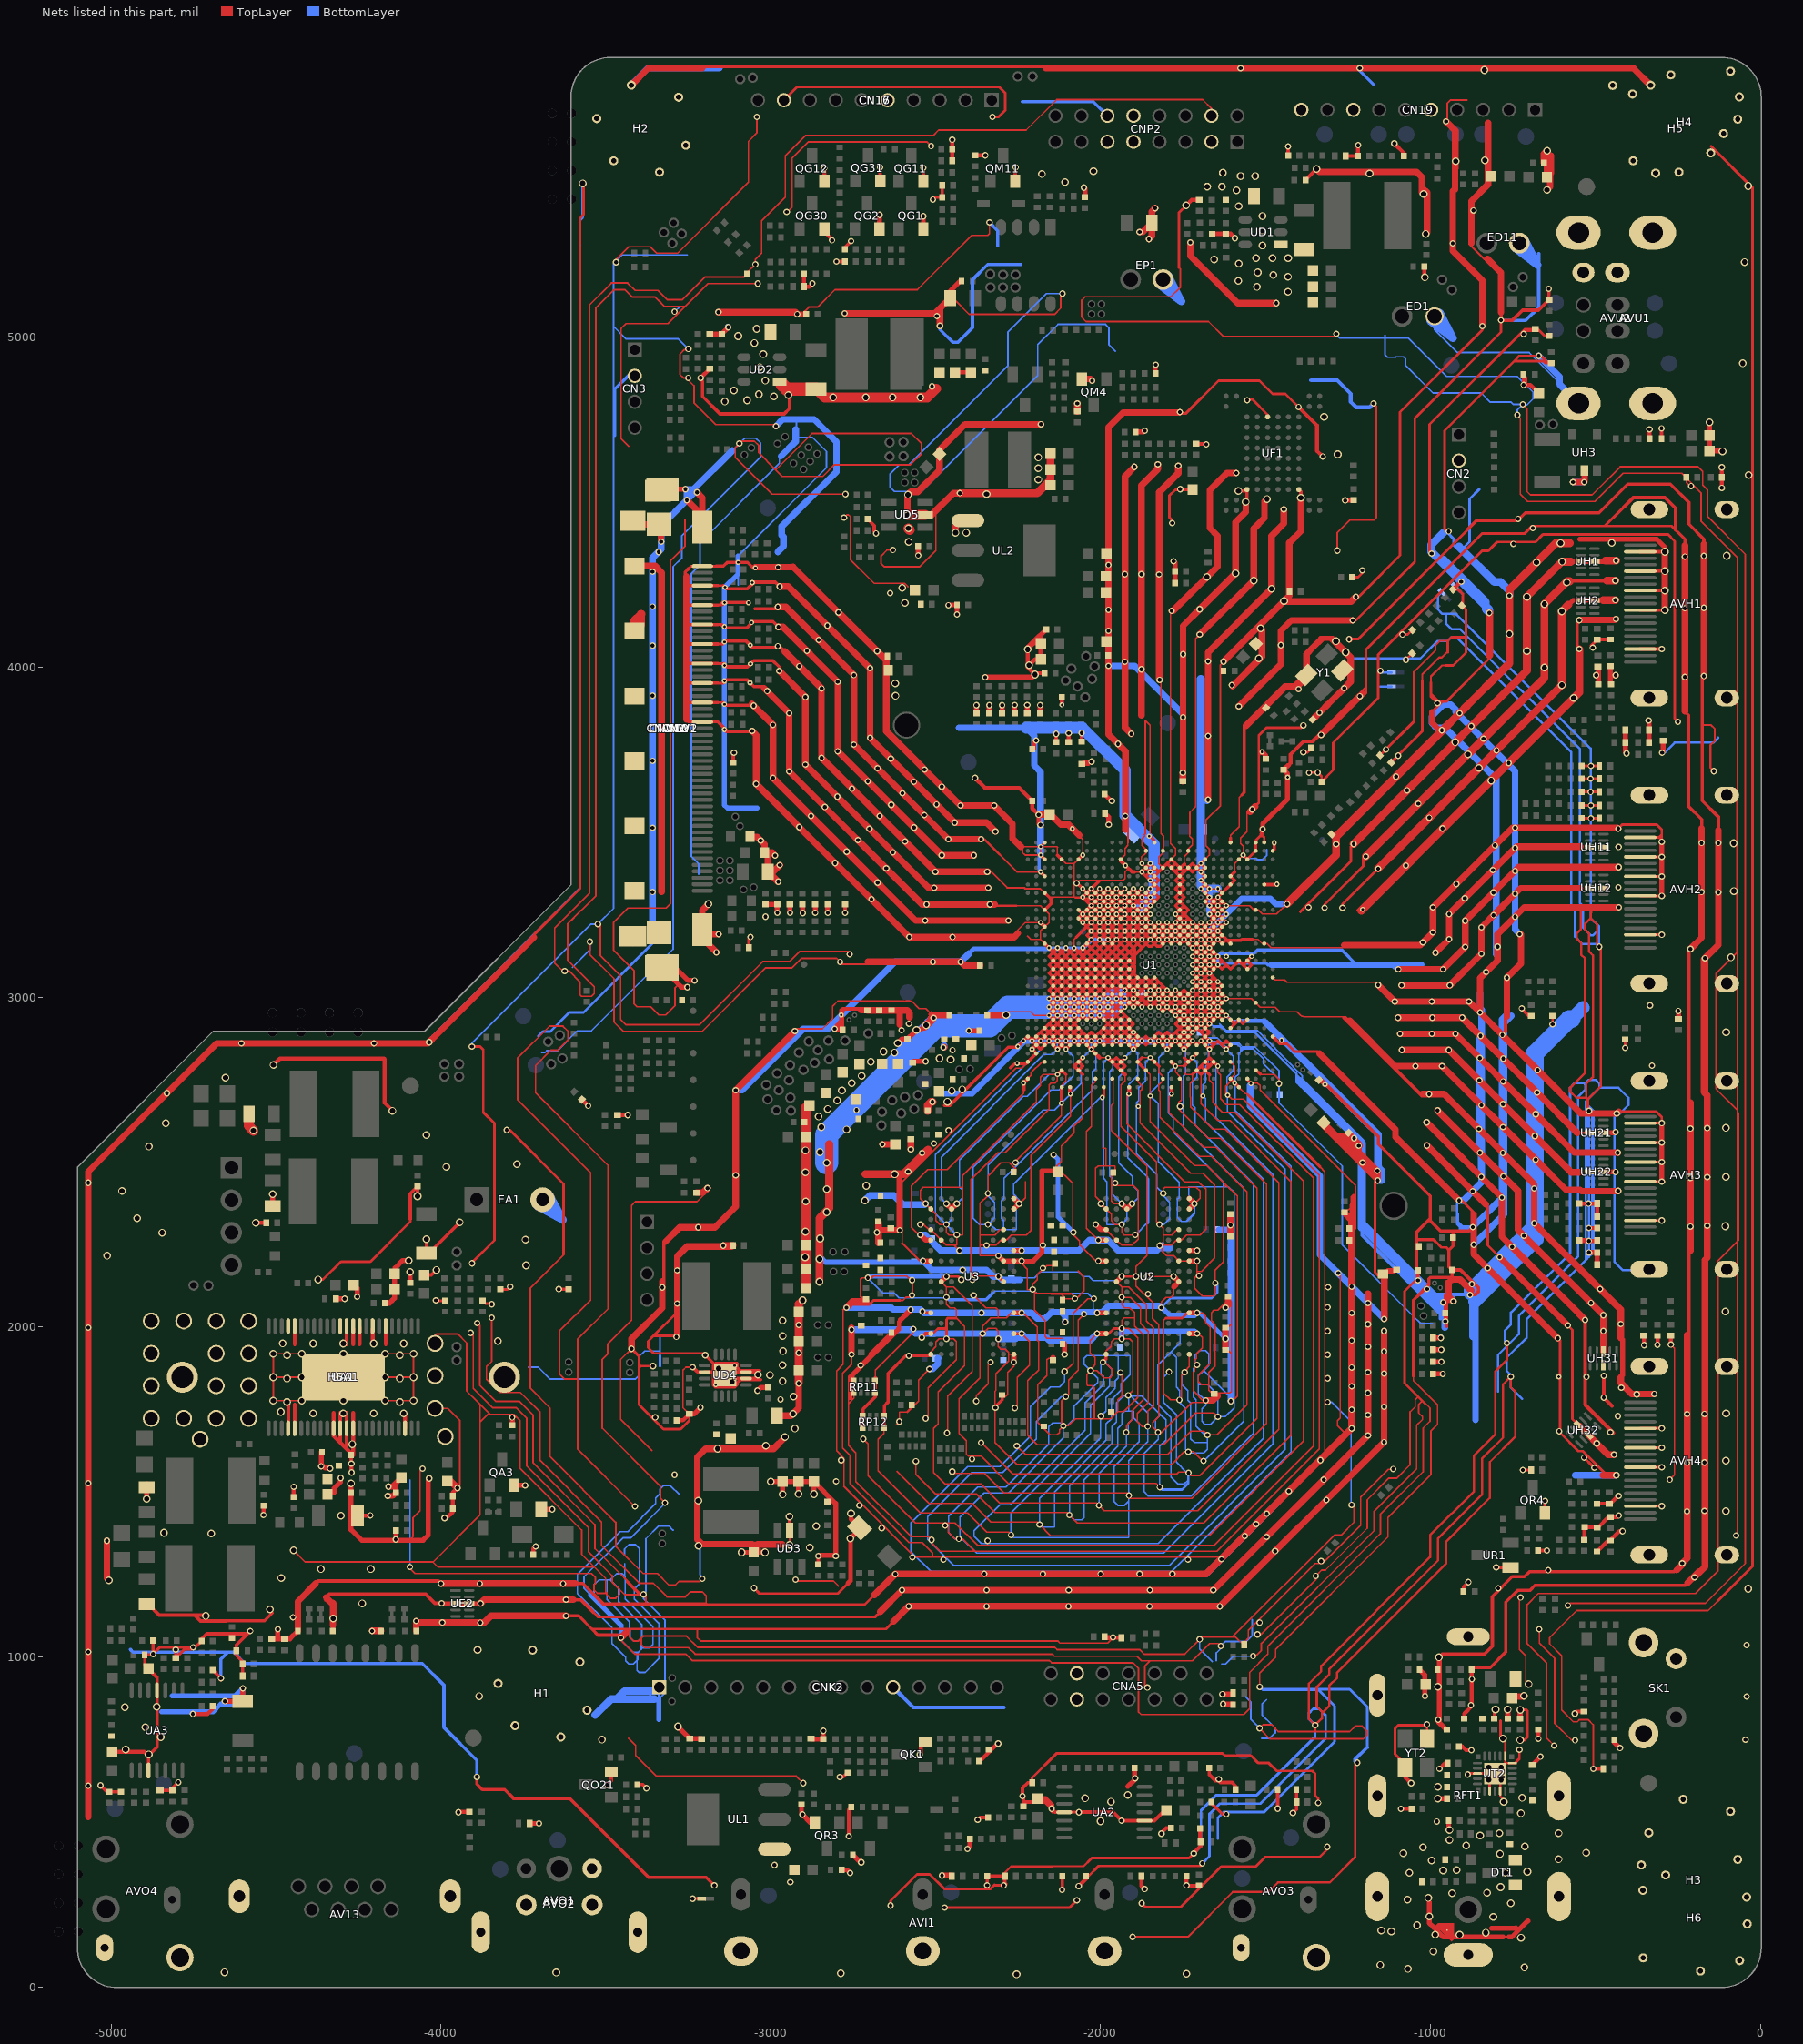
[diagram p0: the nets of this part, all layers, seen from the top]
# Altium PCB MISC86290.PcbDoc (part 19 of 31)
Units mil, origin at the board's own origin, x right, y up, seen from the top; angles counter-clockwise.
Board outline 5104.71 x 5851.49 mil, 2 copper layers (TopLayer, BottomLayer), stack 61.855 mil thick; 1026 components, 667 nets, 4280 pads, 2294 vias.

## Via types
v1: diameter 19.68, hole 11.81, TopLayer to BottomLayer, tented both sides, 1189 vias
v2: diameter 19.68/19.68 (per signal layer), hole 11.81, TopLayer to BottomLayer, tented both sides, 366 vias
v3: diameter 15.75, hole 7.87, TopLayer to BottomLayer, tented both sides, 348 vias
v4: diameter 23.62, hole 15.75, TopLayer to BottomLayer, tented both sides, 309 vias
v5: diameter 15.75/15.75 (per signal layer), hole 7.87, TopLayer to BottomLayer, tented both sides, 59 vias
v6: diameter 24/24 (per signal layer), hole 16, TopLayer to BottomLayer, tented both sides, 23 vias

## Nets (pads, with @x,y where several pads share a name; then routed paths per layer and width w, separated by ;. In a path a pad name is that pad's centre, name@x,y a point inside that pad or via, vN(x,y) a via of type N, cw(c..) or ccw(c..) an arc to the next point about the centre after c; other vN are vias at no path point) (continued)
GND: (continued)
  TopLayer w20: -5069.17,514.17 -5069.17,1454 ; -5069.17,1476.08 -5069.17,1454 ; v1(-5069.17,1998) -5069.17,1929 ; -5069.17,2424 -5069.17,2408 ; v1(-5013,1352) -5013,1238 v4(-5007,1232) ; CE4.1@-4433.73,1078.79 -4433.73,1168.21 -4379.78,1222.16 ; -4348.5,1180 -4330.79,1162.29 -4327.42,1162.29 ; -4327.42,1094.52 -4327.42,1162.29 ; -4327.42,1164.08 -4327.42,1162.29 ; v4@-4326,1126 -4326,1162.29 -4327.42,1162.29 ; v1(-4209.16,1078.06) -4208.44,1078.79 CE2.1@-4181.46,1078.79 ; CE1.1@-4075.03,1078.77 v1(-4075.03,1108.52) ; -4065.5,1103.5 -3869.21,1103.5 -3848.55,1124.16 v2(-3621.16,1124.16) ; v2(-4000,1222.16) v2(-3882,1222.16) -3593.16,1222.16 ; CA21.1@-3981,1533 -3971.35,1533 -3950.35,1512 v1(-3950,1512) ; v1(-3880,1162) -3868.84,1173.16 -3598,1173.16 ; -3717.86,3181.26 -4014.61,2884.5 v1(-4035.91,2863.2) -4039.22,2859.89 -4680,2859.89 -5069.17,2470.72 -5069.17,2408 ; v1(-3454.25,1058) -3444.25,1068 -3433.75,1078.5 ; H2.3@-3423.23,5764.76 -3372.04,5815.96 -3208,5815.96 ; v1(-3422.5,1934) -3422.5,1964 -3329,2057.5 -3329,2138.75 ; CNW12.59@-3413.37,3322.4 CNW12.59@-3413.37,3322.4 ; CNW12.58@-3413.37,3519.25 CNW12.58@-3413.37,3519.25 ; CNW12.57@-3413.37,3716.1 CNW12.57@-3413.37,3716.1 ; CNW12.54@-3413.37,4306.65 -3350.9,4306.65 -3331,4286.75 -3331,3319.72 ; CNW3.53@-3407.27,4433.42 CNW2.53@-3338.37,4433.42 CNW2.53@-3362.25,4409.55 ; v1@-3333,4384.87 CNW2.53@-3333,4418 ; -3319.25,2258.5 -3275.75,2302 -3169,2302 -3106.41,2364.59 ; v1@-3287.25,1972.84 -3284,1976.09 -3284,2214 -3253.84,2244.16 CD39.1@-3117.93,2244.16 ; -3256,3841.75 -3256,4275.75 ; v1@-3254,4506 CNW12.52@-3207.67,4459.67 ; CNW12.52@-3227.9,4445 CNW12.52@-3207.67,4424.76 CNW12.52@-3207.67,4459.67 ; D5.A@-3225,2407.27 -3205.73,2407.27 v1(-3192,2421) ; v1(-3223.9,4530.21) -3207.67,4513.97 CNW12.52@-3207.67,4459.67 ; CNW12.60@-3194.71,3204.29 CNW12.60@-3207.67,3204.29 ; v4(-3189,3282) -3207.67,3263.33 CNW12.60@-3207.67,3204.29 ; v1(-3165,3136) -3207.67,3178.67 CNW12.60@-3207.67,3204.29 ; v1(-3159,5076.61) -2926.11,5076.61 v1(-2920,5070.5) ; v1(-3158.5,3190.5) -3193.88,3190.5 CNW12.60@-3207.67,3204.29 ; v1(-3144.16,2247) CD39.1@-3114.98,2247 ; -3106.41,2436 -3106.41,2364.59 ; RW56.1@-3063.22,3486 -3042,3486 v1(-3030.5,3474.5) -3019.22,3463.22 RW55.1@-3019.22,3438 -2996.5,3438 v1(-2987.5,3429) ; v1@-3057.25,3889 v1(-2993.75,3825.5) v1(-2993.75,3664.68) v1(-2770.07,3441) -2561.18,3232.11 v1(-2280.13,3232.11) ; v1(-3057,3807) -3044.75,3794.75 v1(-3044.75,3646.38) v1(-2805,3406.64) v1(-2580.47,3182.11) v1(-2449,3182.11) ; v3@-3047,4303.5 -2933.02,4303.5 -2932.02,4303.5 ; CD21.1@-3040,1326 -3056,1342 -3209,1342 -3223,1356 -3223,1606 -3198.32,1630.68 -2992.32,1630.68 v4(-2957,1666) ; -3040,1341 -2966,1341 ; -3020.25,3937 v1(-2944.25,3861) v1(-2944.25,3684.48) -2540.88,3281.11 v1(-2336,3281.11) -2322.13,3281.11 ; RW55.1@-3008.97,3427.75 CM18.2@-3008.97,3380.5 ; CD33.2@-2979.62,1731.23 -2938.77,1731.23 -2915.57,1754.43 v1(-2915.57,1829) C61.1@-2915.57,1867.63 ; v1(-2979.25,4183) -2954.86,4183 v1(-2748.25,3976.39) v1(-2748.25,3765.66) v1(-2461.7,3479.11) v1(-2362.86,3479.11) ; v1@-2978.47,3350 CM18.2@-3008.97,3380.5 ; v1(-2977.25,4122) -2963.16,4122 v1(-2797.25,3956.09) v1(-2797.25,3745.37) v1(-2481.99,3430.11) v1(-2385,3430.11) ; v1(-2974.31,3989.07) v1(-2895.25,3910) v1(-2895.25,3704.77) -2521.58,3331.11 v1(-2341,3331.11) ; v1(-2973.25,4245) -2947.25,4245 v1(-2699.25,3997) v1(-2699.25,3785.96) v1(-2442.4,3529.11) -2346.21,3529.11 v1(-2319.13,3502.03) ; v1(-2973,3400.5) -2993,3380.5 CM18.2@-3008.97,3380.5 ; -2957.85,4047.4 v1(-2846.25,3935.79) v1(-2846.25,3725.07) v1(-2501.29,3380.11) ; -2932.52,4304 -2932.02,4303.5 ; v1(-2927.12,2897.12) v1(-3106.41,2717.84) v1(-3106.41,2460) -3106.41,2364.59 ; -2908.52,4280 -2932.02,4303.5 ; v1(-2776,5072.86) -2502.42,5072.86 CM17.2@-2456.28,5119 -2492.42,5082.86 ; v2@-2770.67,2060.23 -2752.86,2078.03 C102.1@-2711.21,2078.03 ; -2725.75,2960.5 C11.1@-2707.95,2960.5 ; -2718.63,2960.5 C11.1@-2707.95,2960.5 ; -2705.41,3106.84 -2705.25,3107 v1(-2509,3107) v1(-2424.51,3107) -2413.51,3096 C5.2@-2365.73,3096 ; -2694.72,1916.42 C80.1@-2632.87,1978.27 ; -2685.75,1188.25 v1(-2622.89,1251.11) -2524.11,1251.11 -1680.52,1251.11 v2(-1529,1402.63) v2(-1429.63,1502) -1257.32,1674.32 v1(-1239.22,1692.41) v1(-1239.22,2122.5) -1239.22,2136 ; C69.1@-2674.12,2255.51 -2673.81,2255.83 v2@-2673.81,2292.91 ; C71.1@-2673.81,2318.19 v2@-2673.81,2292.91 ; -2668.1,1136.6 v1(-2602.59,1202.11) -2544.41,1202.11 -2503.82,1202.11 -2086,1202.11 ; v1(-2661.81,2553.69) C37.2@-2623,2553.69 ; -2650.25,3858 -2650.25,3806.25 ; -2627.95,1107.45 v1(-2582.3,1153.11) ; v2@-2610.81,2292.91 v2@-2673.81,2292.91 ; -2609.16,2917.16 -2609.16,2953.34 ; v4(-2586,4461) -2586,4521.5 v4(-2584.5,4523) -2576.15,4531.35 -2554.74,4531.35 -2488.83,4597.25 -2488.83,4659.07 -2411.13,4736.78 v1(-2181.22,4736.78) ; -2580,2938.5 -2580,2953 -2586.57,2959.57 C11.1@-2707.03,2959.57 C11.1@-2707.95,2960.5 ; v1(-2575.5,2538.5) C77.1@-2575.5,2569 ; UD5.2@-2531.88,4462.5 -2511.83,4462.5 -2446.55,4527.78 v1(-2427,4527.78) ; -2512.97,2948.03 -2510.97,2946.03 R45.1@-2466.97,2946.03 ; v1(-2487.25,5035) -2487.25,5081 ; v1@-2475,2848 v1@-2474.76,2848.24 ; v4@-2440,4410 -2440,4429 -2424.02,4444.98 UL2.1@-2402.27,4444.98 ; -2403.96,3182.11 v1(-2449,3182.11) ; v1(-2344,3380.11) v1(-2501.29,3380.11) ; v1@-2341.86,3380.11 v1(-2501.29,3380.11) ; -2334.04,2946.03 v6(-2286.72,2946.03) ; -2250.75,3193.45 -2262.08,3182.11 -2272.65,3182.11 v1(-2449,3182.11) ; -2242.27,3456.23 -2267.19,3481.16 -2267.19,3525.31 v1(-2323,3581.11) v1(-2425.1,3581.11) -2650.25,3806.25 ; v1@-2188.98,3553.26 -2153.63,3553.26 -2150.72,3553.26 -2121.21,3523.75 -2098.2,3523.75 -2064.84,3490.39 ; -2166,5815.96 -1509.5,5815.96 ; v1(-2098,1153.11) -2087,1153.11 ; v1(-2097,1202.11) -2086,1202.11 ; C17.2@-2071,4775.73 v1(-2071,4800) ; QM4.E@-2057.75,4874 -2031,4874 v1(-2026,4869) ; -1976.78,3955.89 C16.1@-1976.78,4214.44 ; -1976.45,4381 C21.1@-1976.45,4349 ; -1926,3979.11 -1926,4187.16 ; -1925.13,3508.11 -1925.13,3745.13 -1976.45,3796.45 v1(-1976.45,4004.31) C21.1@-1976.45,4349 ; v1(-1907.63,3798.37) -1926.45,3817.2 -1926.45,4578.87 v1(-1897.75,4607.57) ; v1(-1882,5319.42) -1872.55,5319.42 CP1.1@-1844.97,5347 ; -1876.45,3854.31 -1876.45,4077 ; v1(-1876.45,3994) -1876.45,4077 ; v1(-1854.08,5298.24) -1844.97,5307.36 CP1.1@-1844.97,5347 ; v1(-1834.9,5391.9) -1844.97,5381.82 CP1.1@-1844.97,5347 ; v1(-1826.75,4615.11) -1826.75,4600.98 -1876.45,4551.27 -1876.45,4077 ; v1@-1823,3963.75 -1823,4193 ; -1823,4163.75 -1823,4193 ; v1(-1785,4171) -1780.36,4171 -1757.68,4193.68 ; -1774.21,4177.16 -1757.68,4193.68 ; v1(-1764.75,4611.11) -1764.75,4588.36 -1823,4530.11 -1823,4193 ; v1(-1760,4773.5) -1761.5,4772 -1931.75,4772 -1976.45,4727.3 -1976.45,4475 C21.1@-1976.45,4349 ; C18.2@-1751,3654.73 v1(-1751,3680) ; v1@-1750.25,3680.47 -1750.25,4125.75 v1(-1699.93,4176.07) v4(-1591.25,4284.75) -1591.25,4440.11 -1560.25,4471.11 v4(-1560.25,4501.11) ; v1(-1728.25,5288) -1728.25,5247.25 -1585,5104 v1(-1468,5104) ; v2(-1699.87,4099.13) v4(-1536.25,4262.75) ; v2(-1681.42,1777.17) -1659.72,1777.17 C74.1@-1646.36,1790.53 ; v1(-1674.72,3598.03) -1674.72,4045.28 v4(-1482.25,4237.75) ; -1646.25,4389 -1646.25,4359 ; v2(-1627.47,4017.53) v4@-1521,4124 ; R67.1@-1621.38,1936.93 C99.1@-1621.38,1991.42 ; R62.1@-1606.61,2281.42 C70.1@-1606.61,2335.91 ; v2@-1600.18,3943.18 -1511,4032.35 -1511,4114 v4@-1521,4124 ; v1(-1589.25,4589.11) -1617.25,4589.11 -1669.25,4537.11 -1669.25,4421.91 -1646.25,4398.91 -1646.25,4359 ; v1(-1581.47,3881.27) -1454,4008.74 -1454,4084 ; v1@-1570,5815.96 -1509.5,5815.96 ; -1559.47,3822.66 -1440.63,3941.5 -1425,3941.5 ; v1@-1547.32,3562.51 v1(-1540.72,3569.11) -1531.92,3577.92 ; -1536.25,4317 v4(-1536.25,4262.75) ; -1503.27,4489.11 -1503.27,4453.09 ; v4(-1496.25,4510.11) -1503.27,4503.09 -1503.27,4453.09 ; -1482.25,4263 v4(-1482.25,4237.75) ; v1(-1454,4067) -1454,4084 ; v1(-1444.77,4478.63) -1444.77,4435.59 -1482.25,4398.11 v4(-1482.25,4237.75) ; v4@-1437.11,4199.11 -1355,4199.11 ; v1(-1400,3934) -1407.5,3941.5 -1425,3941.5 ; -1393.25,4463.11 -1393.25,4412.11 ; v4(-1393.25,4514.11) -1393.25,4412.11 ; C57.2@-1357.39,3841.45 v1@-1342.42,3856.42 ; C57.2@-1351.23,3847.61 v1@-1342.42,3856.42 ; v4@-1346,5510.27 -1337.23,5501.5 -1042,5501.5 -1025.5,5485 -1025.5,5453.68 ; -1336.52,2828.89 -1106.5,2598.87 -1106.5,2576.25 -931,2400.75 ; v1(-1331.71,3795) v1(-1214.36,3912.36) ; -1331.27,4085.11 -1354.41,4061.97 -1376.34,4040.02 Y1.4@-1376.34,3977.04 -1411.86,3941.5 -1425,3941.5 ; -1319.17,3879.67 -1297.92,3900.92 ; -1297.11,4085.11 -1242,4030 -1242,3956.84 v1(-1261.92,3936.92) -1297.92,3900.92 ; -1293.22,4199.11 -1355,4199.11 ; -1269.61,4142.11 -1283,4142.11 ; -1262.34,3157.85 -1251.27,3157.85 -1031.15,3157.85 v1(-1023,3166) v1(-993,3196) v1@-993,3202 ; C13.2@-1260.94,2345.88 -1239.22,2324.17 -1239.22,2312 ; -1245,2928.31 -1107.54,2790.85 v1(-964.96,2790.85) v1(-681.3,2507.2) -589.61,2415.5 -546.66,2415.5 -542.66,2411.5 -432.5,2411.5 v1(-431.66,2412.34) ; -1239.22,2137.11 -1239.22,2312 ; -1238.5,2539.5 -1228.14,2539.5 -1212.64,2524 ; v1(-1236,4142.11) -1283,4142.11 ; -1235.75,2368.25 -1235.75,2315.48 -1239.22,2312 ; v1@-1230.13,4210.13 -1241.15,4199.11 -1355,4199.11 ; v1(-1217.82,2549.62) -1217.82,2529.18 -1212.64,2524 ; -1189.72,2101.11 v1(-1189.72,2072.5) v1(-1189.72,1671.24) v2(-1323.97,1537) v2(-1497,1363.97) v1(-1658.86,1202.11) -2086,1202.11 ; v1(-1160.5,2444) -1160.5,2471.86 -1212.64,2524 ; v1(-1158.58,3036.85) -1131.86,3010.14 ; v1@-1151.92,3030.19 -1131.86,3010.14 ; -1140.72,1679 v1(-1140.72,1650.94) ; -1140.72,1975 -1140.72,1958 ; v1(-1140.72,1987.8) -1140.72,1958 ; v1(-1140.72,2024) -1140.22,2024.5 -1140.22,2143.19 -1139.22,2144.19 -1139.22,2160.53 C201.1@-1138.85,2160.9 ; v1(-1098.58,2937.85) v1(-904.07,2937.85) v1(-677.03,2710.82) -555.22,2589 ; v1(-1097.72,3084.85) v1(-961.99,3084.85) v1(-895,3151.84) ; v1(-1092.58,2888.85) v1(-924.36,2888.85) v1(-681.01,2645.49) -564.51,2529 -432.05,2529 v1(-432.53,2528.53) ; v1(-1088,3035.85) v1(-941.69,3035.85) v1(-846,3131.54) v1(-846,3211.3) -798.15,3259.15 ; v1(-1087.25,2839.85) v1(-944.66,2839.85) v1(-683.9,2579.1) -573.81,2469 -548,2469 ; -1076.5,2986.85 v1(-1108.58,2986.85) ; -1024.65,2706.16 -959.08,2706.16 ; v4(-1021,5435) -1025.5,5439.5 -1025.5,5453.68 ; v4(-1015,5314) -1010.75,5318.25 -1010.75,5438.93 -1025.5,5453.68 ; v1(-1012.01,2620.49) v1(-783.59,2392.08) -783.59,2273.83 v1(-752.88,2243.12) -566.88,2057.12 ; v1(-1010.9,2550.1) -832.59,2371.78 ; v1(-1004.5,2706.16) -959.08,2706.16 ; -993,3206 v1@-993,3202 ; v1(-984.85,3134.85) v1(-944,3175.7) v1(-944,3251.89) -739.7,3456.18 -545,3456.18 ; -979.09,3286.09 v1(-993,3272.19) ; v1(-978.61,2656.39) -734.59,2412.37 -734.59,2294.12 v1(-717.07,2276.6) -532.73,2092.27 ; v1(-953,5655) -925.15,5627.15 -925.15,5513.15 -926,5512.31 -926,5448.7 ; -950.57,2420.46 v1(-913.55,2383.45) ; -932.96,5332 -932.96,5262.25 ; v1(-930.63,2078.13) -944.84,2092.34 -944.84,2134.26 -935.26,2143.84 -909.71,2143.84 -876.5,2110.63 ; -926,5463.77 -926,5450.59 -932.96,5443.63 -932.96,5262.25 ; -895,3191 v1(-895,3151.84) ; -875.96,5318 -875.96,5285.86 -875.96,5413.06 -825.53,5463.48 -825.53,5649.87 ; -869.59,2339.48 -869.59,2221.23 ; -859,2210.64 -869.59,2221.23 ; -850,3276.59 v1(-895,3231.59) ; v1(-843.25,5034.03) -843.25,5154 ; -843.25,5099.2 -843.25,5154 ; -827.55,5237.45 -786.25,5196.16 ; v1(-809.1,3248.19) -798.15,3259.15 ; -793,3195 -797,3191 ; v1(-790.53,2211.47) v1(-584,2004.94) ; -786.25,5075.59 -786.25,5150 ; -768.5,2941.84 v1(-768.5,3058.89) -725.84,3101.55 ; CT30.1@-750.17,880.02 -717.98,880.02 v4(-716.58,881.42) ; v1(-730,3191) -726.84,3191 -725.84,3190 -725.84,3101.55 ; -725.84,3141 -725.84,3101.55 ; CU14.1@-656.44,5529 -656.44,5556.48 v4(-646.93,5566) ; CU16.1@-647.36,5486 -647.36,5547.41 ; v4(-647,5447) -637.44,5456.56 CU16.1@-637.44,5486 ; CU16.1@-635.58,5497.78 -635.58,5550.84 ; v1(-614.18,1965.82) v1(-827.18,2178.82) -869.59,2221.23 ; v1(-568,4561.43) v1(-534,4561.43) -533,4562.43 UH3.2@-533,4596.87 ; UH32.GND@-551.03,1701.87 UH32.GND@-522.08,1672.92 v1(-496.33,1647.17) -461.99,1612.83 v2(-443.74,1612.83) ; -547,3330 -727.3,3330 -798.15,3259.15 ; v1@-542.25,4143.87 -440.38,4143.87 v2(-438.11,4146.14) ; v1@-534.76,2025 -566.88,2057.12 ; v1(-531.5,2021.74) -566.88,2057.12 ; v1(-513.23,2072.77) -532.73,2092.27 ; v1(-486.09,2114.91) -500.59,2129.41 ; -476.66,1550.66 v2(-437,1550.66) ; UH31.GND@-476.26,1925.42 -476.26,1944 ; -476.26,1955 -476.26,1944 ; v1(-476,1988) -476,1972.26 -476.26,1972 ; v1(-431,3511) -433.5,3513.5 -751.68,3513.5 v1(-993,3272.19) ; v1(-430,3394) -732.59,3394 v1(-895,3231.59) ; v1(-429.68,3272) -513,3272 -538.34,3272 -716,3272 -797,3191 ; v1@-429.22,2653 -434.72,2647.5 v1(-435.5,2647.5) -519.69,2647.5 -544.42,2647.5 v1(-675.71,2778.79) v1(-782.46,2885.54) v1(-850.23,2953.31) ; -423.5,1848 -423.5,1830.5 -390,1797 v1(-322,1797) ; -423.5,1966.81 -423.5,2052.33 -500.59,2129.41 ; -385.12,5815.96 H5.3@-333.93,5764.76 ; -383.87,5815.96 -1509.5,5815.96 ; v4(-289.88,4173.23) v4(-289.88,4232.29) v4(-289.88,4291.34) v4(-289.88,4350.4) ; -254.15,1262.75 -237,1279.9 v1(-237,1284) -222.16,1298.84 -222.16,1976.09 ; -229,3866.1 v1(-229,3970.5) v1(-229,4179) v1(-229,4335.5) -229,4370 ; -220.21,1224.57 -186,1258.78 -186,1255 ; -212.16,2231.19 -212.16,2680.81 ; v1(-212.16,3145.95) -178.5,3179.61 v1(-178.5,3318.5) v1(-178.5,3467.5) -178.5,3511.53 ; v1(-200,1241) -186,1255 ; v1(-171.5,3973.5) v1(-171.5,4180) v1(-171.5,4337.5) -171.5,4373 ; -127.5,3506.5 v1(-127.5,3467.5) -127.5,3158.48 v1(-168,3117.98) ; AVH1.23@-103.22,4468.97 AVH1.23@-103.22,4478.35 ; -5069.17,1454 -5069.17,1929 ; -5069.17,1929 -5069.17,2408 ; -2932.02,4303.5 -2650.25,4021.72 -2650.25,3806.25 ; v1(-2582.3,1153.11) -2553,1153.11 ; v1(-2582.3,1153.11) -2564.71,1153.11 -2553,1153.11 ; -2553,1153.11 -2483.52,1153.11 -2087,1153.11 ; -2087,1153.11 v1(-1638.56,1153.11) v2(-1471,1320.67) v2(-1316,1475.67) v1(-1140.72,1650.94) ; -1757.68,4193.68 -1646.25,4305.12 -1646.25,4359 ; v4(-1536.25,4262.75) -1536.25,4420.11 -1503.27,4453.09 ; v4@-1521,4124 -1428.25,4216.75 -1428.25,4377.11 -1393.25,4412.11 ; -1454,4084 -1454,4110.39 -1422.28,4142.11 -1283,4142.11 ; v1@-1342.42,3856.42 -1297.92,3900.92 ; v1(-1140.72,1650.94) -1140.72,1958 ; -1131.86,3010.14 v1(-1108.58,2986.85) ; v1(-1108.58,2986.85) v1(-883.77,2986.85) v1(-850.23,2953.31) ; v1@-993,3202 v1(-993,3272.19) ; -959.08,2706.16 -685.59,2432.67 v1(-685.59,2420) v1(-685.59,2314.42) -500.59,2129.41 ; -932.96,5262.25 -843.25,5172.55 -843.25,5154 ; v1(-895,3151.84) v1(-895,3231.59) ; v1(-850.23,2953.31) -850.23,3057.77 -797,3111 v1(-797,3153) -797,3191 ; -786.25,5150 -786.25,5196.16 ; -786.25,5150 -786.25,5170 -786.25,5196.16 ; -532.73,2092.27 v1(-476.26,2035.79) -476.26,1972 ; -476.26,1944 -476.26,1972 ; -186,1255 -168,1273 -168,2203.22 -161.16,2210.06 v1(-161.16,2307) v1(-161.16,2454.5) v1(-161.16,2603) -161.16,2701.94 -168,2708.78 ; -168,2708.78 -171.16,2711.94 -171.16,3114.83 v1(-168,3117.98) ; -168,2708.78 v1(-168,3117.98)
  TopLayer w24: v1(-2915.57,1829) -2915.57,2069.43 v6(-2904,2081) ; v6@-2852.97,2138.51 -2852.97,2168 ; v6@-2852.97,2142.03 -2852.97,2168 ; -2822.97,2554.03 -2822.97,2360.03 -2852.97,2330.03 -2852.97,2168 ; -2712.66,2463.03 -2610.81,2463.03 -2597.97,2463.03 -2522.97,2538.03 ; v6@-2534,2910 -2512.97,2931.03 v1@-2512.97,2934.03 ; C49.1@-2524.46,2656 -2524.46,2672.04 -2514,2682.5 v1(-2510,2682.5) ; v1(-2427,4527.78) -2192.63,4527.78 -2152.26,4568.15 CD54.1@-2152.26,4647.68 ; v1(-1434.96,3282.21) -1286.56,3430.62 v1(-1286.56,3463.5) -1286.56,3486.45 -1186.01,3587 ; v1(-1233.56,3464.5) -1147.53,3550.53 ; v3@-1210.07,3261.57 -1050.35,3421.29 -1050.35,3422.85 ; v1(-1196.56,3426.55) -1158.8,3464.3 ; -1188,3587 -1186.01,3587 ; -1180.56,3442.55 -1158.8,3464.3 ; v1(-1158.57,3389.57) -1088.07,3460.07 ; -1157.53,3540.53 -1147.53,3550.53 ; -1129.55,3493.55 -1116.55,3506.55 ; -1101.57,3446.57 -1088.07,3460.07 ; -1064.1,3409.1 -1050.35,3422.85 ; -888,3885 v1(-912,3861) ; -822,4037.28 v1(-822,4165) ; -582.34,4189.34 v4(-602,4169.68) v4(-602,3946.15) -1088.07,3460.07 ; v4@-578.25,4261 -585.63,4261 v4(-655,4191.63) -655,3968.1 -1116.55,3506.55 ; -578,4376.36 -620.18,4376.36 -761,4235.53 v1(-761,4217) -761,4012.01 v1(-912,3861) ; -575.25,4320 v4@-601.58,4320 ; -575.25,4320.31 v4(-601.27,4320.31) v4@-601.58,4320 ; v1(-549,4055) -549,3924.2 -1050.35,3422.85 ; -476.25,4203.9 v1(-439.65,4203.9) ; -469.25,4323.36 v1(-437.63,4323.36) ; -466.25,4262.96 v1(-439.65,4262.96) ; -1186.01,3587 -965,3808 v1(-912,3861) ; -1158.8,3464.3 -1116.55,3506.55 ; -1147.53,3550.53 -708,3990.06 v4(-708,4213.58) v4@-601.58,4320
  TopLayer w25: -3394.25,4161.09 -3394.25,4128.93 CNW12.55@-3413.37,4109.8 -3413.37,4140.87 -3393.25,4161 ; C12.1@-1323.83,2619.33 -1323.83,2614.13 -1275.2,2565.49 ; -1245.15,2546.15 v1@-1170.34,2471.34 ; -1237.35,2538.35 -1237.35,2527.65 -1235.01,2525.3 ; v1@-1218.12,2549.62 -1234,2565.49 -1275.2,2565.49 ; v1(-1206.37,2498.8) v1@-1206.37,2507.37 ; -1163.5,2453.8 -1235.01,2525.3 ; -1275.2,2565.49 -1235.01,2525.3
  TopLayer w30: CA27.2@-4583.03,2645.5 -4583.03,2610.03 v4(-4568.5,2595.5) ; CD42.1@-2894.97,2126.5 C4.1@-2894.97,2664 ; CD13.1@-2862.79,4843.64 -2837.15,4818 -2787,4818 ; v4@-2821.15,4818 -2787,4818 ; v4@-2584.5,4462.5 UD5.2@-2531.88,4462.5 ; v4(-2583,4421) v4@-2579,4417 ; -2499.25,4844.75 -2526,4818 -2787,4818
  TopLayer w40: UD2.1@-2965.41,4857.59 -2951.47,4843.64 CD13.1@-2862.79,4843.64